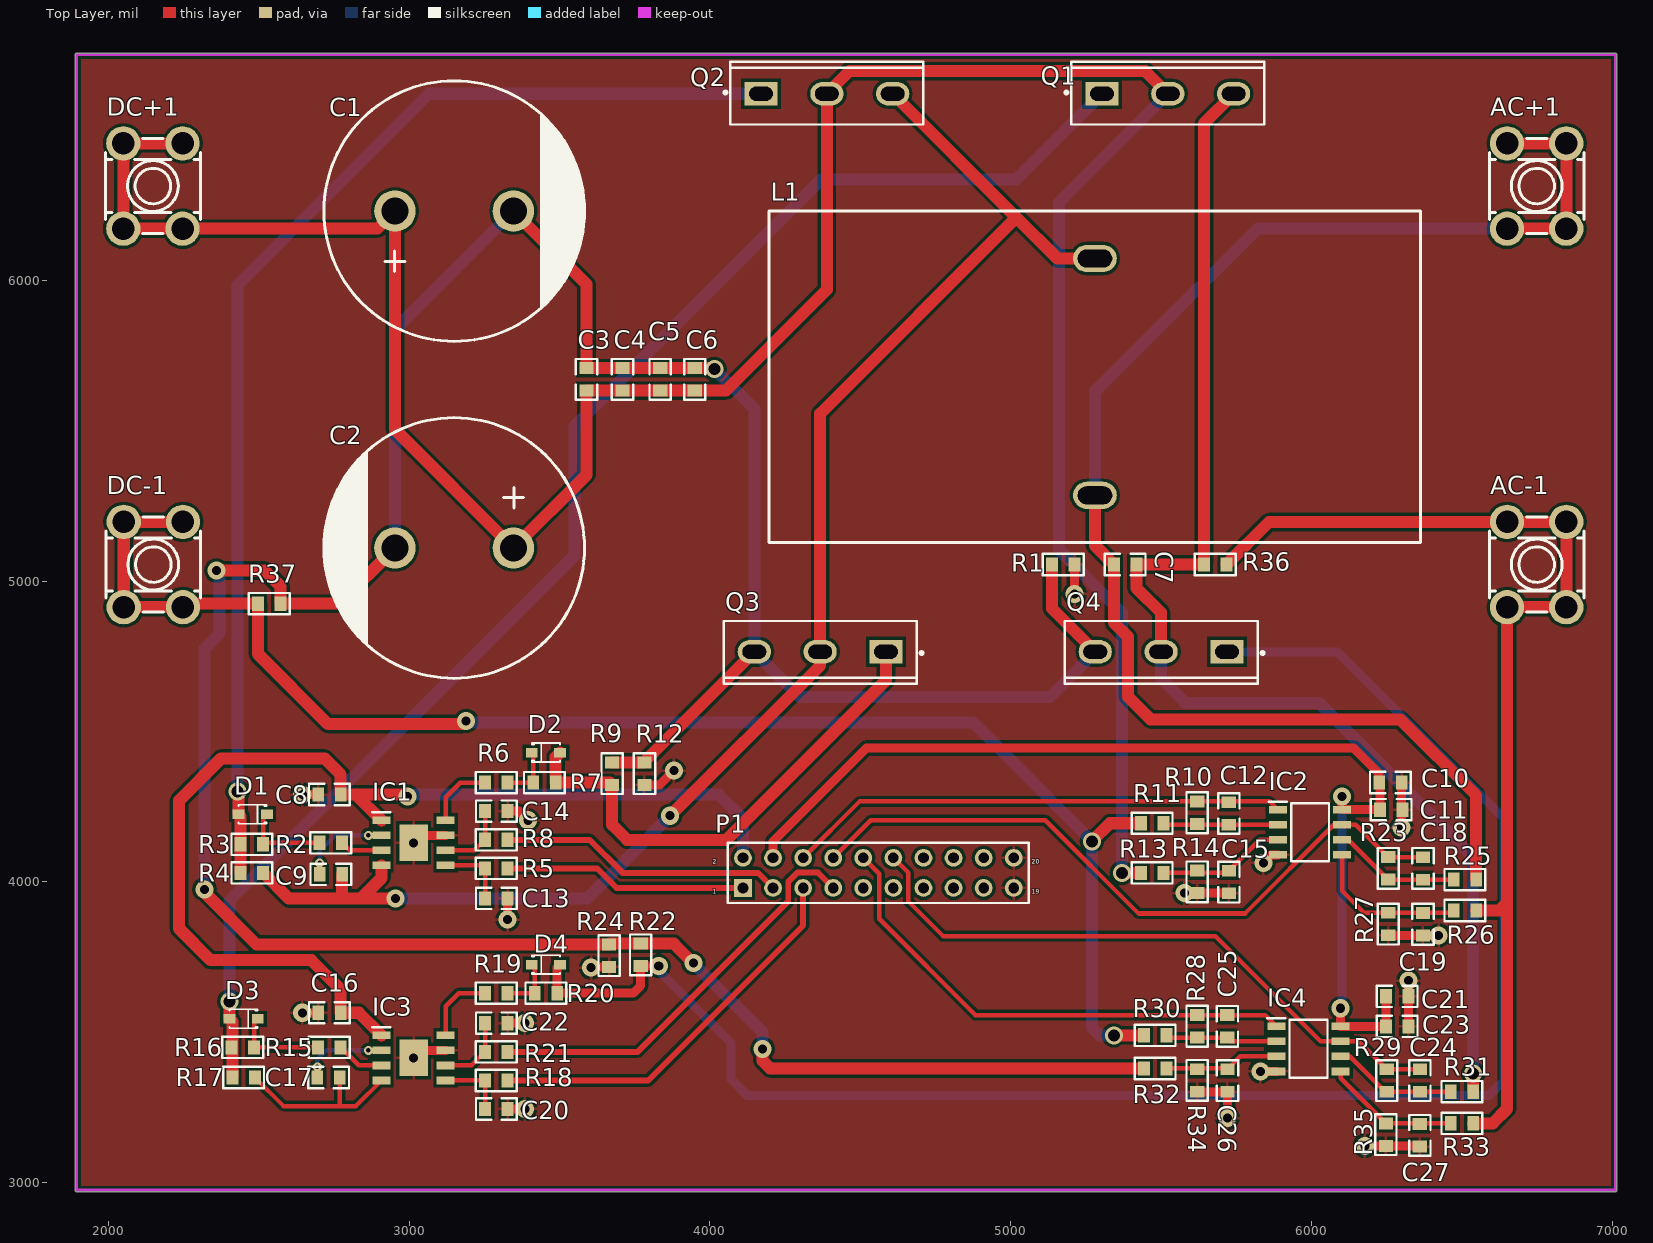
[diagram p0: Top Layer view]
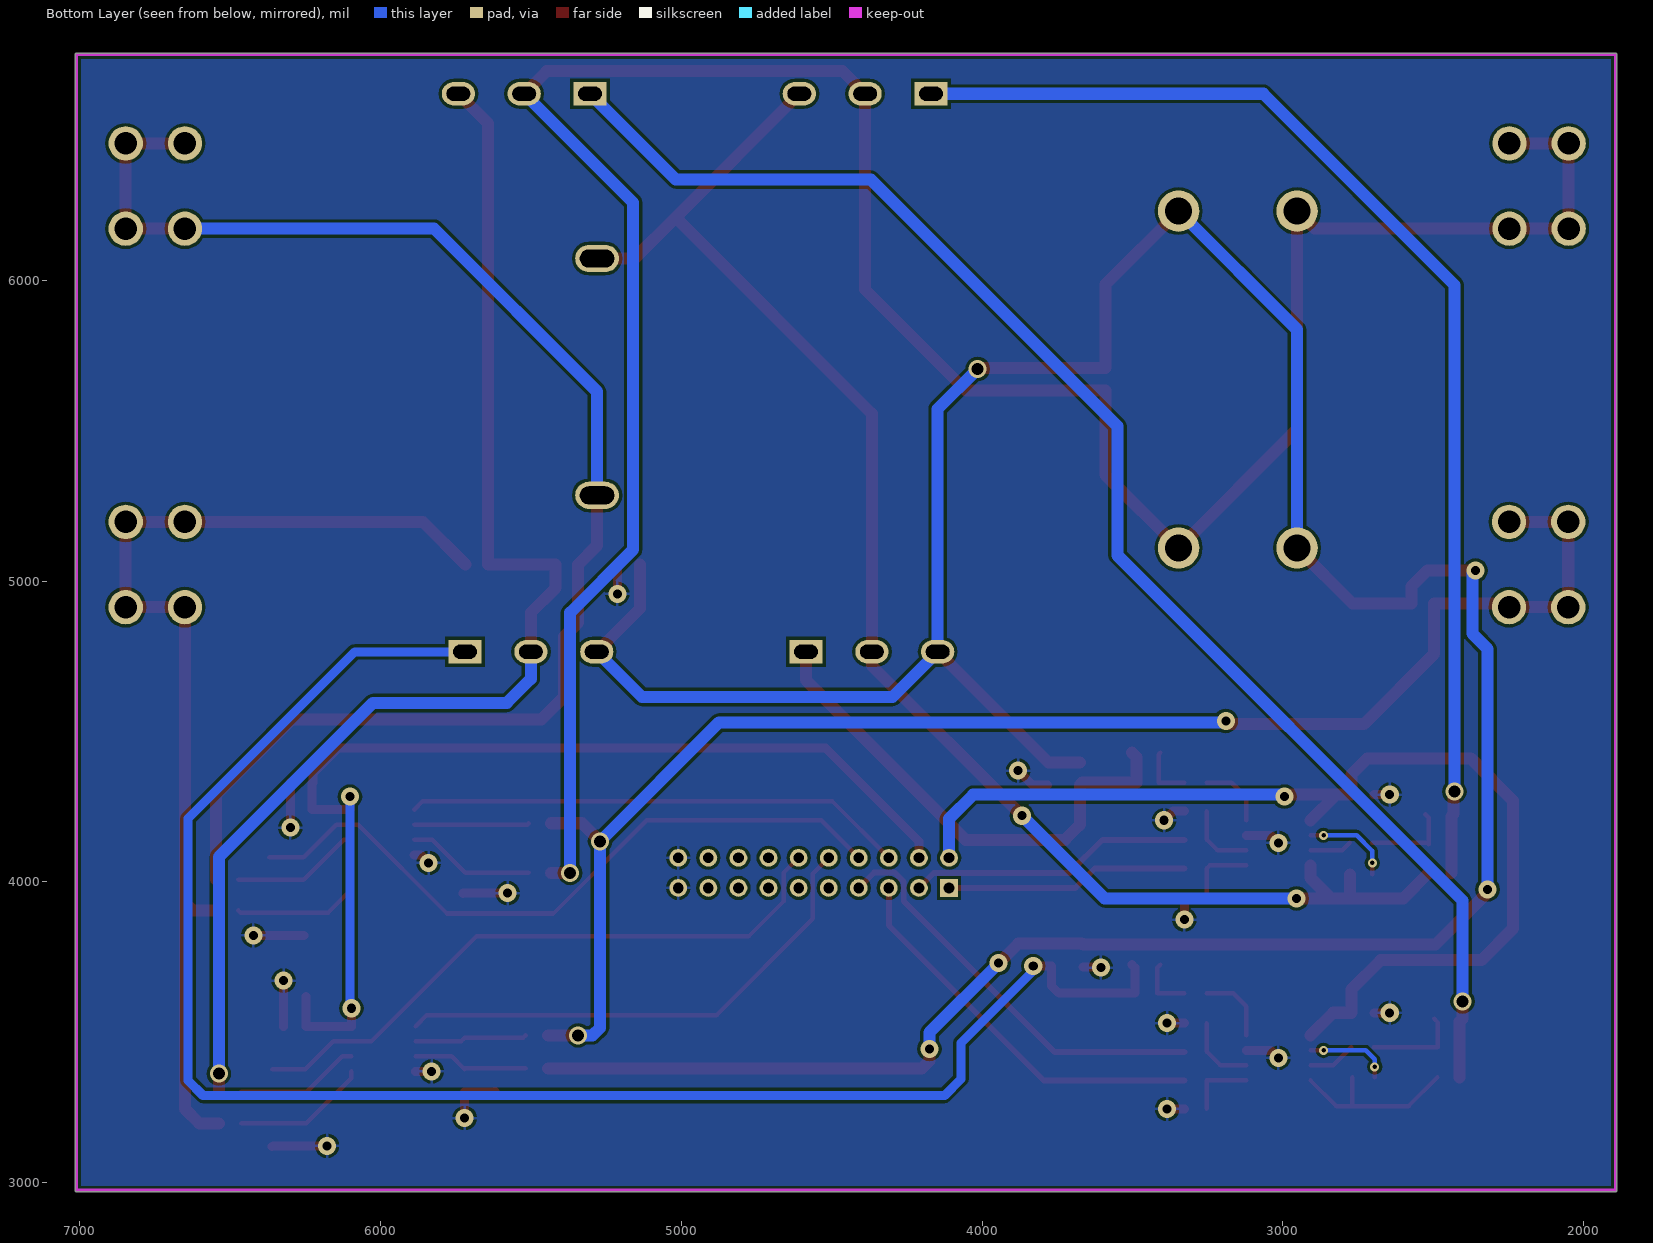
[diagram p1: Bottom Layer view, seen from below]
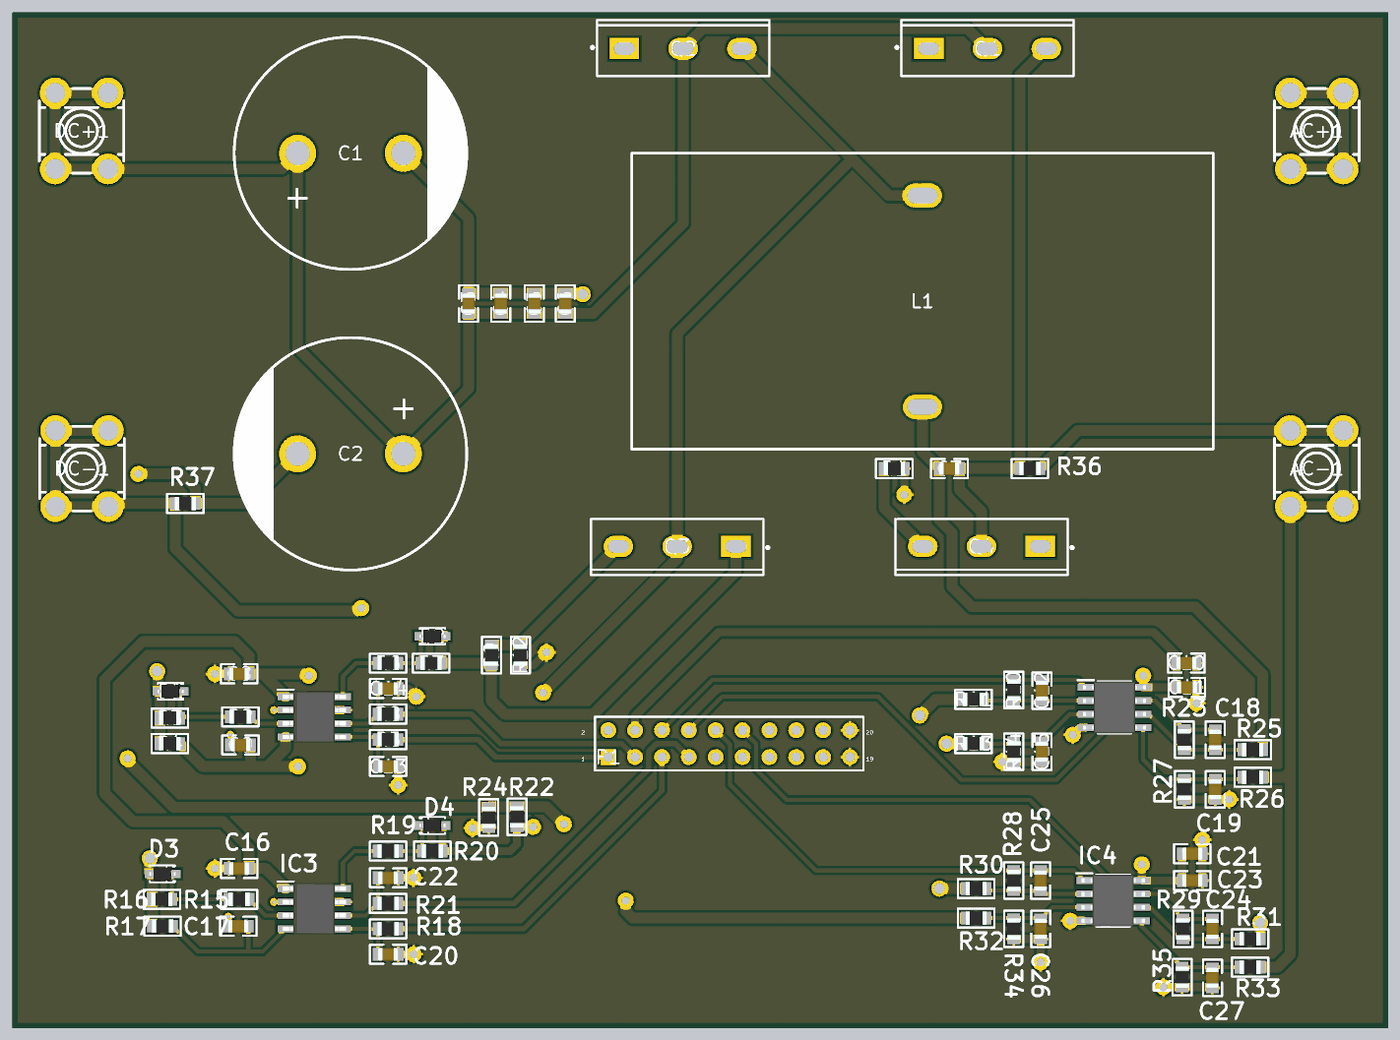
[diagram p2: 3D render of the assembled board from above, using the file's embedded part models]
# Altium PCB MISC82254.PcbDoc
Units mil, origin at the board's own origin, x right, y up, seen from the top; angles counter-clockwise.
Board outline 5125.03 x 3785.03 mil, 2 copper layers (Top Layer, Bottom Layer); 82 components, 45 nets, 220 pads, 41 vias.

## Layer stack, top to bottom (the 12.6 mil dielectric is the usual default, probably not edited)
Top Solder: solder mask 0.4, Solder Resist, Dk 3.5
Top Layer: signal copper 1.4
Dielectric 1: dielectric 12.6, FR-4, Dk 4.8
Bottom Layer: signal copper 1.4
Bottom Solder: solder mask 0.4, Solder Resist, Dk 3.5

## Board outline
1895,2969.99 cw(c1895,2975) 1889.98,2975 1889.98,6750 cw(c1895,6750) 1895,6755.02 7010,6755.02 cw(c7010,6750) 7015.02,6750 7015.02,2975 cw(c7010,2975) 7010,2969.99

## Design rules (kind name [scope] priority, off if disabled: settings)
Clearance [All] p1: gap=10
MinimumSolderMaskSliver [All] p1: minsoldermaskwidth=0
PolygonConnect [All] p1: connectstyle=Relief reliefconductorwidth=10 reliefentries=4 polygonreliefangle="90 Angle" airgapwidth=10
RoutingVias [All] p1: holewidth=28 width=50 viastyle="Through Hole" minholewidth=28 minwidth=50 maxholewidth=28 maxwidth=50
SilkToSilkClearance [All] p1: silktosilkclearance=0
SilkToSolderMaskClearance [IsPad] p1: minsilkscreentomaskgap=0 clearancetoexposedcopper=TRUE
SolderMaskExpansion [All] p1: expansion=4
Width [All] p1: maxlimit=60 minlimit=10 preferedwidth=10
27 further rules are at their usual default settings.

## Components (designator, comment, footprint, x,y, rotation, side; value= is the part's Value field where it differs from the comment)
AC+1 "CONnector" CONN-TH_T44001 6748.43,6313.27 r0 top
AC-1 "CONnector" CONN-TH_T44001 6748.43,5055 r0 top
C1 "1000uF/100V" CAPE 3150,6230 r0 top
C2 "1000uF/100V" CAPE 3150,5110 r180 top
C3 "100nF/100V" 0805C 3590,5670 r90 top
C4 "100nF/100V" 0805C 3710,5670 r90 top
C5 "100nF/100V" 0805C 3835,5670 r90 top
C6 "100nF/100V" 0805C 3950,5670 r90 top
C7 "10uF/250V" 0805C 5380,5055 r0 top
C8 "1uF/25V/0603" 0805C 2735,4290 r0 top
C9 "1uF/25V/0603" 0805C 2740,4025 r0 top
C10 "1nF/25V/0805" 0805C 6262.8,4330.55 r180 top
C11 "100nF/25V/0805" 0805C 6265,4240.28 r180 top
C12 "1nF/25V/0805" 0805C 5724.72,4227.8 r270 top
C13 "100pF/25V/0603" 0805C 3290,3945 r0 top
C14 "100pF/25V/0603" 0805C 3290,4235 r0 top
C15 "1nF/25V/0805" 0805C 5725,4000 r270 top
C16 "1uF/25V/0603" 0805C 2735,3564.72 r0 top
C17 "1uF/25V/0603" 0805C 2732.01,3349.72 r0 top
C18 "1nF/25V/0805" 0805C 6370,4045 r270 top
C19 "1nF/25V/0805" 0805C 6370,3860 r270 top
C20 "100pF/25V/0603" 0805C 3290,3245 r0 top
C21 "1nF/25V/0805" 0805C 6285,3620 r180 top
C22 "100pF/25V/0603" 0805C 3290,3530 r0 top
C23 "100nF/25V/0805" 0805C 6285,3520 r180 top
C24 "1nF/25V/0805" 0805C 6360,3340 r270 top
C25 "1nF/25V/0805" 0805C 5719.72,3520 r270 top
C26 "1nF/25V/0805" 0805C 5720.28,3340 r270 top
C27 "1nF/25V/0805" 0805C 6359.72,3157.8 r270 top
D1 "?" SOD-323 2480,4225 r0 top
D2 "?" SOD-323 3455,4430 r180 top
D3 "?" SOD-323 2450,3545 r0 top
D4 "?" SOD-323 3455,3725 r180 top
DC+1 "CONnector" CONN-TH_T44001 2148.63,6313.27 r180 top
DC-1 "CONnector" CONN-TH_T44001 2150,5055 r0 top
IC1 "UCC27211AQDDARQ1" "SOIC8 Powerpad" 3015,4130 r0 top
IC2 "OPA2350UA" SOIC127P600X175-8N 5995,4165 r0 top
IC3 "UCC27211AQDDARQ1" "SOIC8 Powerpad" 3015,3415 r0 top
IC4 "OPA2350UA" SOIC127P600X175-8N 5990,3445 r0 top
L1 "Inductor" IND-TH_L55.0-W28.0-P20.00-D1.3 5280,5678.7 r0 top
P1 "Header 10X2" HDR2X10 4110,3980 r0 top
Q1 "IPW60R037CSFD" TO-247-3_L15.9-W5.1-P5.44-L 5522.3,6620 r0 top
Q2 "IPW60R037CSFD" TO-247-3_L15.9-W5.1-P5.44-L 4388.84,6620 r0 top
Q3 "IPW60R037CSFD" TO-247-3_L15.9-W5.1-P5.44-L 4366.54,4765 r180 top
Q4 "IPW60R037CSFD" TO-247-3_L15.9-W5.1-P5.44-L 5500,4765 r180 top
R1 "0R/1206" 0805R 5175,5055.28 r0 top
R2 "2R/0603" 0805R 2740,4130 r180 top
R3 "2R/0603" 0805R 2477.6,4125 r180 top
R4 "10k/0603" 0805R 2477.6,4030 r180 top
R5 "100R/0603" 0805R 3290,4045 r180 top
R6 "2R/0603" 0805R 3290,4330 r0 top
R7 "2R/0603" 0805R 3450,4330 r0 top
R8 "100R/0603" 0805R 3290,4140 r180 top
R9 "10k/0603" 0805R 3675,4360 r270 top
R10 "15k/0805" 0805R 5620,4230 r90 top
R11 "402k/0805" 0805R 5470,4195 r0 top
R12 "1R/0603" 0805R 3782.64,4360 r90 top
R13 "402k/0805" 0805R 5470,4030 r0 top
R14 "15k/0805" 0805R 5620,4000 r90 top
R15 "2R/0603" 0805R 2735,3450 r180 top
R16 "2R/0603" 0805R 2447.4,3450 r180 top
R17 "10k/0603" 0805R 2450,3350 r180 top
R18 "100R/0603" 0805R 3290,3340 r180 top
R19 "2R/0603" 0805R 3290,3630 r0 top
R20 "2R/0603" 0805R 3455,3630 r0 top
R21 "100R/0603" 0805R 3290,3435 r180 top
R22 "10k/0603" 0805R 3770,3757.4 r270 top
R23 "15k/0805" 0805R 6255,4045 r90 top
R24 "1R/0603" 0805R 3665,3755 r90 top
R25 "402k/0805" 0805R 6510,4007.6 r0 top
R26 "402k/0805" 0805R 6510,3905 r0 top
R27 "15k/0805" 0805R 6255,3860 r90 top
R28 "15k/0805" 0805R 5620,3520 r90 top
R29 "15k/0805" 0805R 6250,3339.61 r90 top
R30 "402k/0805" 0805R 5480,3490 r0 top
R31 "402k/0805" 0805R 6500,3302.6 r0 top
R32 "402k/0805" 0805R 5480,3380 r0 top
R33 "402k/0805" 0805R 6500,3197.4 r0 top
R34 "15k/0805" 0805R 5620,3340 r90 top
R35 "15k/0805" 0805R 6247.2,3160 r90 top
R36 "0R/1206" 0805R 5680,5055 r180 top
R37 "0R/1206" 0805R 2535,4925 r180 top

## Footprints (in the part's own frame and the unit in brackets; to place one, negate y for a bottom-side part, rotate by r counter-clockwise, add the part's x,y. Pads: shape width x height; smd on the part's side, far side on the other; paste and mask are expansions set on the pad)
0805C [mm]
  rect 1x1.2 smd: 1(-0.94,0.007) 2(0.96,0.007)
  silkscreen extent -1.72,-0.89 1.74,0.91, body extent -1,-0.63 1,0.63, height 1.45
0805R [mm]
  rect 1x1.2 smd: 1(-0.95,0) 2(0.95,0)
  silkscreen extent -1.73,-0.9 1.73,0.9, body extent -1,-0.64 1,0.64, height 0.65
CAPE [mm]
  round 3.5 hole 2.3: 1(-5,0) 2(5,0)
  silkscreen extent -11,-11 11,11
CONN-TH_T44001 [mm]
  round 2.9 hole 1.9: 0(-2.5,-3.6) 0(-2.5,3.6) 0(2.5,-3.6) 0(2.5,3.6)
  silkscreen extent -4,-4 4,4
HDR2X10 [mm] "Connector; Header; 10x2 Position"
  rect 1.5x1.5 hole 0.9: 1(0,0)
  round 1.5 hole 0.9: 2(0,2.54) 3(2.54,0) 4(2.54,2.54) 5(5.08,0) 6(5.08,2.54) 7(7.62,0) 8(7.62,2.54) 9(10.16,0) 10(10.16,2.54) 11(12.7,0) 12(12.7,2.54) 13(15.24,0) 14(15.24,2.54) 15(17.78,0) 16(17.78,2.54) 17(20.32,0) 18(20.32,2.54) 19(22.86,0) 20(22.86,2.54)
  silkscreen extent -1.27,-1.27 24.13,3.81
IND-TH_L55.0-W28.0-P20.00-D1.3 [mm]
  oval 3.7x2.3 hole 1.5 slot 2.9 at 0 deg paste-2539.97 mask+0.05: 1(0,10) 2(0,-10)
  silkscreen extent -27.5,-14 27.5,14
SOD-323 [mm]
  rect 1x0.8 smd: 1(1.2,0) 2(-1.2,0)
  silkscreen extent -1.2,-0.8 1.2,0.8, body extent -1.24,-0.63 1.24,0.62, height 0.93
"SOIC8 Powerpad" [mm]
  rect 1.525x0.65 smd: 1(-2.712,1.905) 2(-2.712,0.635) 3(-2.712,-0.635) 4(-2.712,-1.905) 5(2.712,-1.905) 6(2.712,-0.635) 7(2.712,0.635) 8(2.712,1.905)
  rect 2.4x3.1 smd: 9(0,0)
  silkscreen extent -3.47,2.58 -1.95,2.58, body extent -3,-2.45 3,2.45, height 1.57
SOIC127P600X175-8N [mm]
  rect 1.525x0.65 smd: 1(-2.712,1.905) 2(-2.712,0.635) 3(-2.712,-0.635) 4(-2.712,-1.905) 5(2.712,-1.905) 6(2.712,-0.635) 7(2.712,0.635) 8(2.712,1.905)
  silkscreen extent -3.47,-2.45 1.6,2.58, body extent -3,-2.45 3,2.45, height 1.75
TO-247-3_L15.9-W5.1-P5.44-L [mm]
  rect 2.8x2 hole 1.2 slot 2 at 0 deg: 1(-5.56,0)
  oval 2.8x2 hole 1.2 slot 2 at 0 deg: 2(0,0) 3(5.56,0)
  silkscreen extent -8.69,-2.6 8.15,2.7

## Part data
C1 C2 C3 C4 C5 C6 C7 C8 C9 C10 C11 C12 C13 C14 C15 C16 C17 C18 C19 C20 C21 C22 C23 C24 C25 C26 C27: library part CAP
D1 D2 D3 D4: library part DIODE_1
IC1 IC2 IC3 IC4: "Integrated Circuit"
P1: "Header, 10-Pin, Dual row"
R1 R2 R3 R4 R5 R6 R7 R8 R9 R10 R11 R12 R13 R14 R15 R16 R17 R18 R19 R20 R21 R22 R23 R24 R25 R26 R27 R28 R29 R30 R31 R32 R33 R34 R35 R36 R37: library part Resistor, "Resistor"

## Via types
v1: diameter 60, hole 30, Top Layer to Bottom Layer, 30 vias
v2: diameter 60, hole 40, Top Layer to Bottom Layer, 7 vias
v3: diameter 30, hole 15, Top Layer to Bottom Layer, 4 vias

## Nets (pads, with @x,y where several pads share a name; then routed paths per layer and width w, separated by ;. In a path a pad name is that pad's centre, name@x,y a point inside that pad or via, vN(x,y) a via of type N, cw(c..) or ccw(c..) an arc to the next point about the centre after c; other vN are vias at no path point)
5V: C10.2 C11.2 C21.2 C23.2 IC2.8 IC4.8 P1.4 | length 3539
  Top Layer w30: P1.4 4210,4135 4520,4445 6140,4445 6225,4360 C10.2 6227.2,4328.07 C11.2 IC2.8 v1(6101.77,4283.23) ; v1(6096.77,3580) IC4.8 6246.93,3520 C23.2 C21.2
  Bottom Layer w30: v1(6096.77,3580) 6101.77,3585 v1(6101.77,4283.23)
+12V: C8.2 C16.2 IC1.1 IC3.1 P1.2 | length 3605
  Top Layer w40: IC3.1 2833.23,3565 C16.2 2772.8,3642.2 2675,3740 2340,3740 2235,3845 2235,4270 2375,4410 2720,4410 2772.8,4357.2 C8.2 2822.95,4290.28 ; IC1.1 2822.95,4290.28 ; v1(2995,4283.23) 2987.95,4290.28 2822.95,4290.28
  Bottom Layer w40: v1@2995,4280 v1(2995,4283.23) 3001.77,4290 4030,4290 4110,4210 P1.2
g1: D1.2 Q2.1 R3.2 R4.2 | length 3963.3
  Top Layer w40: v2@2432.76,4302.24 D1.2 2440.2,4217.56 R3.2 R4.2
  Bottom Layer w40: v2(2430,4300) 2430,5985 3065,6620 Q2.1
g2: D2.2 Q3.1 R7.2 R9.2 | length 1674.8
  Top Layer w40: D2.2 3487.4,4415.16 R7.2 3667.6,4330 R9.2 3675,4190 3725,4140 4055,4140 4585.44,4670.44 Q3.1
G3: D3.2 Q1.1 R16.2 R17.2 | length 4855.4
  Top Layer w40: v2(2402.76,3602.76) D3.2 2412.6,3535.16 R17.2
  Bottom Layer w40: v2(2402.76,3602.76) 2402.76,3937.76 3550,5085 3550,5515 4370,6335 5018.4,6335 Q1.1
G4: D4.2 Q4.1 R20.2 R22.2 | length 5630.9
  Top Layer w30: D4.2 3492.4,3715.16 R20.2 3745,3630 3770,3655 R22.2 v1(3830,3720) v1@3840,3720
  Bottom Layer w30: v1(3830,3720) 3830,3705 4070,3465 4070,3345 4125,3290 6590,3290 6640,3340 6640,4210 6085,4765 Q4.1
IAC+: AC-1.0 R26.2 R33.2 R36.1 | length 3582
  Top Layer w40: R36.1 5859.13,5196.73 6650,5196.73 6846.85,5196.73 6846.85,4913.27 6650,4913.27 6650,3930 ; R33.2 6602.4,3197.4 6650,3245 6650,3930 ; R26.2 6625,3905 6650,3930
IAC-: C7.2 Q1.3 Q4.2 R31.2 R36.2 | length 4307.9
  Top Layer w40: Q4.2 5500,4895 5417.8,4977.2 C7.2 5642.32,5055.28 R36.2 5642.6,6521.4 Q1.3 ; R31.2 v2(6537.4,3362.6)
  Bottom Layer w40: Q4.2 5500,4675 5580,4595 6025,4595 6537.4,4082.6 v2(6537.4,3362.6)
IAC_ADC: C24.1 IC4.7 P1.12 R29.2 | length 2097.1
  Top Layer w15: P1.12 4660,4030 4660,3935 4775,3820 5680,3820 6030,3470 IC4.7 6157.01,3470 R29.2 C24.1
IDC+: C1.2 C2.2 C3.2 C4.2 C5.2 C6.2 Q3.3 Q4.3 R1.1 R9.1 R12.2 R22.1 R24.2 R32.1 R37.1 | length 10826.1
  Top Layer w40: v1(2320,3975) 2320,3965 2492.6,3792.4 R24.2 3667.4,3794.8 R22.1 3880.2,3794.8 v1(3945,3730) ; v1(2360,5035) 2520,5035 2572.4,4982.6 R37.1 2768.15,4925 C2.2 ; C1.2 3589.72,5987.13 C3.2 C4.2 C5.2 C6.2 4012.2,5707.8 v2(4015,5705) ; R9.1 3780.04,4397.4 Q3.3 ; v1(4175,3445) 4175,3405 4200,3380 R32.1 ; R1.1 5137.6,4908.5 Q4.3
  Bottom Layer w40: v1(2320,3975) 2320,4775 2370,4825 2370,5025 v1(2360,5035) ; C2.2 2953.15,5836.3 C1.2 ; v1(3945,3730) 4175,3500 v1(4175,3445) ; v2(4015,5705) 4147.64,5572.36 Q3.3 4297.63,4615 5131.1,4615 Q4.3
IDC-: DC-1.0 R11.1 R30.1 R37.2 | length 5127.7
  Top Layer w40: DC-1.0@2248.42,5196.73 2051.57,5196.73 2051.57,4913.27 2248.42,4913.27 2260.15,4925 R37.2 2497.6,4757.4 2730,4525 3180,4525 v1(3190,4535) ; v2(5270,4135) 5330,4195 R11.1 ; v2(5342.99,3490) R30.1
  Bottom Layer w40: v1(3190,4535) 3195,4530 4875,4530 v2(5270,4135) 5270,3515 5295,3490 v2(5342.99,3490)
IDC_ADC: C25.1 IC4.1 P1.10 R28.2 | length 1693.1
  Top Layer w15: P1.10 4562.97,4027.03 4562.97,3877.03 4882.6,3557.4 R28.2 5845.83,3557.4 IC4.1
NetC9_1: C9.1 IC1.2 | length 304.5
  Top Layer w15: C9.1 v3(2702.99,4062.99) ; v3(2865,4155) IC1.2
  Bottom Layer w15: v3(2702.99,4062.99) 2702.99,4102.99 2755,4155 v3(2865,4155)
NetC12_2: C12.2 IC2.2 R10.1 R11.2 | length 382.9
  Top Layer w15: R11.2 5512.4,4190 C12.2 IC2.2
NetC13_1: C13.1 IC1.5 R5.2 | length 234.9
  Top Layer w15: IC1.5 3242.6,4055 R5.2 3252.99,4044.61 C13.1
NetC14_1: C14.1 IC1.6 R8.2 | length 240.8
  Top Layer w15: IC1.6 3217.6,4105 R8.2 3252.6,4234.88 C14.1
NetC15_1: C15.1 IC2.3 R13.2 R14.2 | length 426.4
  Top Layer w15: R13.2 5718.27,4030 C15.1 5828.27,4140 IC2.3
NetC17_1: C17.1 IC3.2 | length 285.7
  Top Layer w15: C17.1 v3(2695,3385) ; v3(2865,3440) IC3.2
  Bottom Layer w15: v3(2695,3385) 2695,3410 2725,3440 v3(2865,3440)
NetC18_2: C18.2 IC2.6 R23.1 R25.1 | length 425.7
  Top Layer w15: IC2.6 6122.6,4140 R23.1 R25.1
NetC19_1: C19.1 IC2.5 R26.1 R27.2 | length 524
  Top Layer w15: IC2.5 6101.77,3970 6174.37,3897.4 R27.2 6465,3897.4 R26.1
NetC20_1: C20.1 IC3.5 R18.2 | length 225.7
  Top Layer w15: IC3.5 R18.2 3252.99,3339.61 C20.1
NetC22_1: C22.1 IC3.6 R21.2 | length 244.9
  Top Layer w15: IC3.6 3207.6,3390 R21.2 3252.6,3529.88 C22.1
NetC24_2: C24.2 IC4.6 R29.1 R31.1 | length 414.8
  Top Layer w15: IC4.6 6127.4,3420 6245.2,3302.2 R29.1 6462.2,3302.2 R31.1
NetC25_2: C25.2 IC4.2 R28.1 R30.2 | length 374.1
  Top Layer w15: R30.2 5524.8,3482.6 R28.1 5620.39,3482.2 C25.2 5732.2,3470 IC4.2
NetC26_1: C26.1 IC4.3 R32.2 R34.2 | length 384.9
  Top Layer w15: R32.2 5717.56,3380 C26.1 5763.54,3420 IC4.3
NetC27_1: C27.1 IC4.5 R33.1 R35.2 | length 450.3
  Top Layer w15: IC4.5 6096.77,3347.83 R35.2 R33.1
NetD1_1: D1.1 R2.2 R3.1 | length 294.7
  Top Layer w15: D1.1 2515,4212.76 R3.1 2520,4130 R2.2
NetD2_1: D2.1 R6.2 R7.1 | length 187.2
  Top Layer w15: R6.2 R7.1 3412.6,4425.16 D2.1
NetD3_1: D3.1 R15.2 R16.1 | length 312.9
  Top Layer w15: D3.1 2484.8,3532.56 R16.1 R15.2
NetD4_1: D4.1 R19.2 R20.1 | length 189.3
  Top Layer w15: R19.2 R20.1 3417.6,3715.16 D4.1
NetIC1_3: IC1.3 R2.1 | length 141.2
  Top Layer w15: R2.1 2802.4,4105 IC1.3
NetIC1_8: IC1.8 R6.1 | length 227.6
  Top Layer w15: IC1.8 3121.77,4281.77 3170,4330 R6.1
NetIC3_3: IC3.3 R15.1 | length 160.7
  Top Layer w15: R15.1 2832.4,3390 IC3.3
NetIC3_8: IC3.8 R19.1 | length 245.5
  Top Layer w15: IC3.8 3121.77,3586.77 3165,3630 R19.1
PWM1: P1.1 R5.1 | length 809.5
  Top Layer w19.68: R5.1 3625,4045 3690,3980 P1.1
PWM2: P1.3 R8.1 | length 948.9
  Top Layer w19.68: R8.1 3600,4140 3710,4030 4160,4030 P1.3
PWM3: P1.5 R18.1 | length 1320.9
  Top Layer w19.68: R18.1 3795,3340 4310,3855 P1.5
PWM4: P1.7 R21.1 | length 1388.3
  Top Layer w19.68: R21.1 3760,3435 4260.63,3935.63 4260.63,4000.45 4290.81,4030.63 4359.37,4030.63 P1.7
s1: C9.2 IC1.4 L1.1 Q2.3 Q3.2 R4.1 | length 5086.2
  Top Layer w40: R4.1 2600,3945 2775,3945 ; C9.2 2777.8,3947.8 2775,3945 ; IC1.4 2908.23,4013.23 2840,3945 ; v1(2954.72,3945) 2840,3945 ; v1(3867.5,4220) 4366.54,4719.04 Q3.2 4366.54,5556.54 5018.87,6208.87 ; Q2.3 5018.87,6208.87 ; L1.1 5155.34,6072.4 5018.87,6208.87 ; 2775,3945 2840,3945
  Bottom Layer w40: v1(2954.72,3945) 3592.5,3945 v1(3867.5,4220)
S2: C17.2 IC3.4 R17.1 | length 590.5
  Top Layer w15: R17.1 2582.4,3255 2770,3255 ; C17.2 2769.8,3255.2 2770,3255 ; IC3.4 2823.23,3255 2770,3255
SGND: C8.1 C10.1 C11.1 C13.2 C14.2 C15.2 C16.1 C19.2 C20.2 C21.1 C22.2 C23.1 C26.2 C27.2 IC1.7 IC1.9 IC2.4 IC3.7 IC3.9 IC4.4 P1.19 P1.20 R1.2 R12.1 R14.1 R24.1 R27.1 R34.1 R35.1 | length 1941.1
  Top Layer w30: v1(2645,3565) C16.1 ; v1@2655.28,4290.28 C8.1 ; v1(3015,3415) 3040,3440 IC3.7 ; v1(3015,4130) 3040,4155 IC1.7 ; C20.2 v1(3385.28,3245.28) ; C22.2 v1(3384.72,3530.28) ; v1@3327.8,3887.2 C13.2 ; C14.2 3364.72,4235.28 v1(3395,4205) ; v1@3612.6,3717.6 R24.1 ; R12.1 3832.6,4322.6 v1(3880,4370) ; v1(5212.4,4957.6) R1.2 ; v1(5577.4,3962.6) R14.1 5724.88,3962.6 C15.2 ; R34.1 5620.39,3302.2 C26.2 v1@5720.55,3225.55 ; v1(5830,3370) IC4.4 ; v1(5840,4062.99) 5867.01,4090 IC2.4 ; v1(6177.6,3122.6) R35.1 6357.4,3122.6 C27.2 ; R27.1 6369.88,3822.6 C19.2 v1(6422.8,3822.2) ; v1(6299.8,4180.2) C10.1 ; C23.1 C21.1 v1(6322.01,3672.01)
  other v1: 5720,3215 3605,3715 3327.8,3875 2645,4290
Vin+: C1.1 C2.1 C3.1 C4.1 C5.1 C6.1 DC+1.0 Q1.2 Q2.2 R13.1 | length 8988.9
  Top Layer w40: DC+1.0@2247.06,6455 2050.21,6455 2050.21,6171.54 2247.06,6171.54 2894.69,6171.54 C1.1 2953.15,5503.7 C2.1 3589.72,5352.87 C3.1 C4.1 C5.1 C6.1 4052.99,5632.99 4388.84,5968.84 Q2.2 4463.84,6695 5447.3,6695 Q1.2 ; v2(5369.72,4030) R13.1
  Bottom Layer w40: v2(5369.72,4030) 5369.72,4895.28 5160,5105 5160,6257.7 Q1.2
Vin_adc: C12.1 IC2.1 P1.6 R10.2 | length 1667.2
  Top Layer w15: P1.6 4497.4,4267.4 R10.2 5860.83,4267.4 IC2.1
VOUT+: AC+1.0 C7.1 L1.2 R25.2 | length 4905.1
  Top Layer w40: L1.2 5280,5118.27 C7.1 5342.99,4862.01 5390,4815 5390,4615 5465,4540 6295,4540 6547.4,4287.6 R25.2 ; AC+1.0@6650,6171.54 6846.85,6171.54 6846.85,6455 AC+1.0@6650,6455
  Bottom Layer w40: L1.2 5280,5630 5821.54,6171.54 AC+1.0@6650,6171.54
VOUT_ADC: C18.1 IC2.7 P1.8 R23.2 | length 2307.4
  Top Layer w15: P1.8 4535,4205 5115,4205 5425,3895 5778.96,3895 6073.96,4190 IC2.7 6147.4,4190 R23.2 6255.39,4082.01 C18.1
pads on no net: P1.9 P1.11 P1.13 P1.14 P1.15 P1.16 P1.17 P1.18

## Polygon pours and split planes (outlines as drawn)
SGND on Top Layer "G" (solid, remove dead copper, pour order 0): 1305,7180 1465,7340 7175,7340 7175,2825 7220,2780 7160,2720 1595,2720
SGND on Bottom Layer "G" (solid, remove dead copper, pour order 2): 1420,6920 7515,6920 7570,6865 7335,6630 7335,2705 1800,2705 1695,2810

## Keep-outs
Keep-Out Layer:
  lines w10: 1895,3050 1895,6750 5780,6750 ; 1895,3065 1895,2975 7010,2975 7010,6750 5765,6750